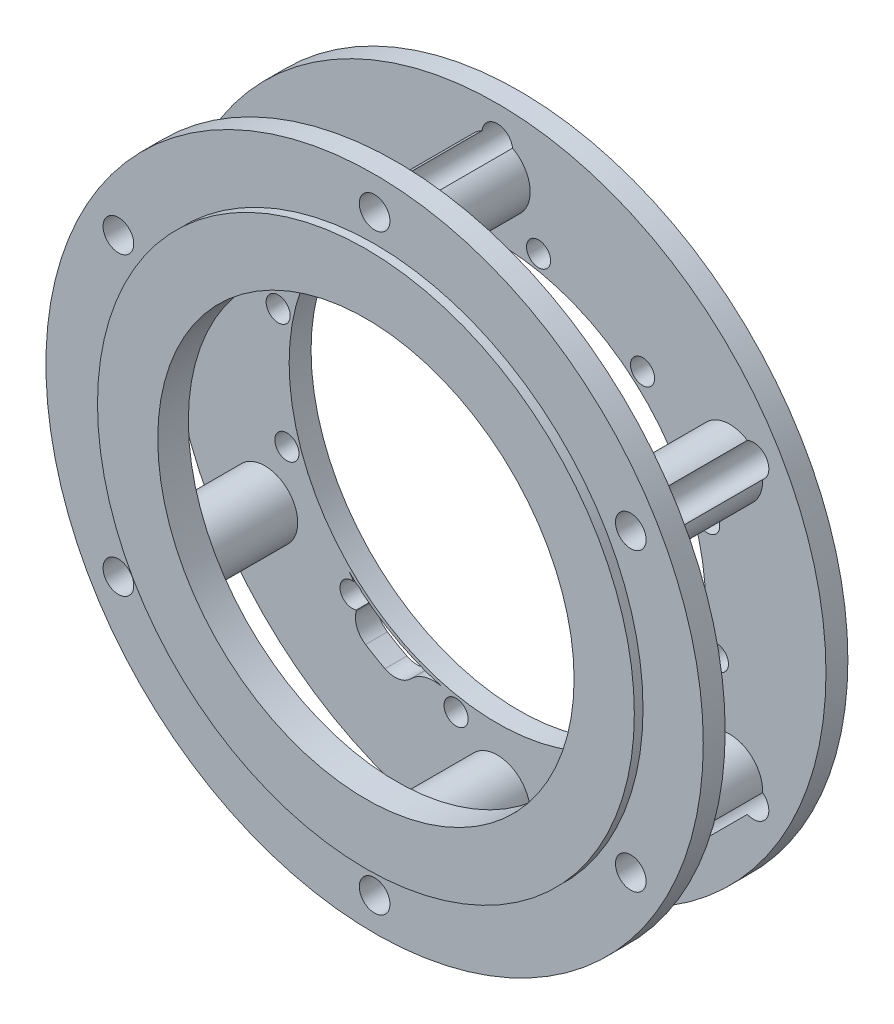
from build123d import *

# Parameters (mm, degrees)
SKETCH1_R           = 150
BOSS_EXTRUDE1_DEPTH = 10
SKETCH2_R           = 15
BOSS_EXTRUDE2_DEPTH = 46
SKETCH3_R           = 150
BOSS_EXTRUDE3_DEPTH = 10
SKETCH4_R           = 122.5
BOSS_EXTRUDE4_DEPTH = 3.96
CUT_EXTRUDE2_REACH  = 225.371
SKETCH5_R           = 7
CUT_EXTRUDE3_REACH  = 225.371
SKETCH6_R           = 95
CUT_EXTRUDE9_DEPTH  = 10
SKETCH8_R           = 5.5
CUT_EXTRUDE10_DEPTH = 10


with BuildPart() as part:
    # Sketch1 → Boss-Extrude1 (new body)
    with BuildSketch(Plane.XY):
        Circle(SKETCH1_R)
    extrude(amount=BOSS_EXTRUDE1_DEPTH)

    # Sketch2 → Boss-Extrude2 (add)
    with BuildSketch(Plane.XY.offset(10)):
        with Locations((0, 122.5)):
            Circle(SKETCH2_R)
        with Locations((106.088111964, 61.25)):
            Circle(SKETCH2_R)
        with Locations((106.088111964, -61.25)):
            Circle(SKETCH2_R)
        with Locations((0, -122.5)):
            Circle(SKETCH2_R)
        with Locations((-106.088111964, -61.25)):
            Circle(SKETCH2_R)
        with Locations((-106.088111964, 61.25)):
            Circle(SKETCH2_R)
    extrude(amount=BOSS_EXTRUDE2_DEPTH)

    # Sketch3 → Boss-Extrude3 (add)
    with BuildSketch(Plane.XY.offset(56)):
        Circle(SKETCH3_R)
    extrude(amount=BOSS_EXTRUDE3_DEPTH)

    # Sketch4 → Boss-Extrude4 (add)
    with BuildSketch(Plane.XY.offset(66)):
        Circle(SKETCH4_R)
    extrude(amount=BOSS_EXTRUDE4_DEPTH)

    # Cut-Extrude2: up to this face of the body (flat: up to its plane)
    cut_extrude2_end = Plane(part.part.faces().sort_by_distance((0, 0, 69.96))[0])
    # Sketch5 → Cut-Extrude2 (cut, up to the picked face)
    with BuildSketch(Plane(origin=(0, 0, 0), x_dir=(-1, 0, 0), z_dir=(0, 0, -1)), mode=Mode.PRIVATE) as cut_extrude2_sk1:
        with Locations((0, 135)):
            Circle(SKETCH5_R)
    cut_extrude2_tool1 = split(extrude(cut_extrude2_sk1.sketch, amount=-CUT_EXTRUDE2_REACH, mode=Mode.PRIVATE), bisect_by=cut_extrude2_end, keep=Keep.BOTH, mode=Mode.PRIVATE)
    # Sketch5 → Cut-Extrude2 (cut, up to the picked face)
    with BuildSketch(Plane(origin=(0, 0, 0), x_dir=(-1, 0, 0), z_dir=(0, 0, -1)), mode=Mode.PRIVATE) as cut_extrude2_sk2:
        with Locations((116.913429511, 67.5)):
            Circle(SKETCH5_R)
    cut_extrude2_tool2 = split(extrude(cut_extrude2_sk2.sketch, amount=-CUT_EXTRUDE2_REACH, mode=Mode.PRIVATE), bisect_by=cut_extrude2_end, keep=Keep.BOTH, mode=Mode.PRIVATE)
    # Sketch5 → Cut-Extrude2 (cut, up to the picked face)
    with BuildSketch(Plane(origin=(0, 0, 0), x_dir=(-1, 0, 0), z_dir=(0, 0, -1)), mode=Mode.PRIVATE) as cut_extrude2_sk3:
        with Locations((116.913429511, -67.5)):
            Circle(SKETCH5_R)
    cut_extrude2_tool3 = split(extrude(cut_extrude2_sk3.sketch, amount=-CUT_EXTRUDE2_REACH, mode=Mode.PRIVATE), bisect_by=cut_extrude2_end, keep=Keep.BOTH, mode=Mode.PRIVATE)
    # Sketch5 → Cut-Extrude2 (cut, up to the picked face)
    with BuildSketch(Plane(origin=(0, 0, 0), x_dir=(-1, 0, 0), z_dir=(0, 0, -1)), mode=Mode.PRIVATE) as cut_extrude2_sk4:
        with Locations((0, -135)):
            Circle(SKETCH5_R)
    cut_extrude2_tool4 = split(extrude(cut_extrude2_sk4.sketch, amount=-CUT_EXTRUDE2_REACH, mode=Mode.PRIVATE), bisect_by=cut_extrude2_end, keep=Keep.BOTH, mode=Mode.PRIVATE)
    # Sketch5 → Cut-Extrude2 (cut, up to the picked face)
    with BuildSketch(Plane(origin=(0, 0, 0), x_dir=(-1, 0, 0), z_dir=(0, 0, -1)), mode=Mode.PRIVATE) as cut_extrude2_sk5:
        with Locations((-116.913429511, -67.5)):
            Circle(SKETCH5_R)
    cut_extrude2_tool5 = split(extrude(cut_extrude2_sk5.sketch, amount=-CUT_EXTRUDE2_REACH, mode=Mode.PRIVATE), bisect_by=cut_extrude2_end, keep=Keep.BOTH, mode=Mode.PRIVATE)
    # Sketch5 → Cut-Extrude2 (cut, up to the picked face)
    with BuildSketch(Plane(origin=(0, 0, 0), x_dir=(-1, 0, 0), z_dir=(0, 0, -1)), mode=Mode.PRIVATE) as cut_extrude2_sk6:
        with Locations((-116.913429511, 67.5)):
            Circle(SKETCH5_R)
    cut_extrude2_tool6 = split(extrude(cut_extrude2_sk6.sketch, amount=-CUT_EXTRUDE2_REACH, mode=Mode.PRIVATE), bisect_by=cut_extrude2_end, keep=Keep.BOTH, mode=Mode.PRIVATE)
    add(cut_extrude2_tool1.solids().sort_by(Axis((0, 135, 0), (0, 0, 1)))[0], mode=Mode.SUBTRACT)
    add(cut_extrude2_tool2.solids().sort_by(Axis((-116.91343, 67.5, 0), (0, 0, 1)))[0], mode=Mode.SUBTRACT)
    add(cut_extrude2_tool3.solids().sort_by(Axis((-116.91343, -67.5, 0), (0, 0, 1)))[0], mode=Mode.SUBTRACT)
    add(cut_extrude2_tool4.solids().sort_by(Axis((0, -135, 0), (0, 0, 1)))[0], mode=Mode.SUBTRACT)
    add(cut_extrude2_tool5.solids().sort_by(Axis((116.91343, -67.5, 0), (0, 0, 1)))[0], mode=Mode.SUBTRACT)
    add(cut_extrude2_tool6.solids().sort_by(Axis((116.91343, 67.5, 0), (0, 0, 1)))[0], mode=Mode.SUBTRACT)

    # Cut-Extrude3: up to this face of the body (flat: up to its plane)
    cut_extrude3_end = Plane(part.part.faces().sort_by_distance((0, 0, 69.96))[0])
    # Sketch6 → Cut-Extrude3 (cut, up to the picked face)
    with BuildSketch(Plane(origin=(0, 0, 0), x_dir=(-1, 0, 0), z_dir=(0, 0, -1)), mode=Mode.PRIVATE) as cut_extrude3_sk1:
        with Locations(Location((0, 0, 0), (0, 0, 180))):
            Circle(SKETCH6_R)
    cut_extrude3_tool1 = split(extrude(cut_extrude3_sk1.sketch, amount=-CUT_EXTRUDE3_REACH, mode=Mode.PRIVATE), bisect_by=cut_extrude3_end, keep=Keep.BOTH, mode=Mode.PRIVATE)
    add(cut_extrude3_tool1.solids().sort_by(Axis((0, 0, 0), (0, 0, 1)))[0], mode=Mode.SUBTRACT)

    # Sketch7 → Cut-Extrude9 (cut)
    with BuildSketch(Plane(origin=(0, 0, 0), x_dir=(-1, 0, 0), z_dir=(0, 0, -1))):
        with BuildLine():
            ThreePointArc((68.235804385, -68.235804384), (48.250000208, -83.571451345), (24.976038317, -93.211842112))
            ThreePointArc((24.976038317, -93.211842112), (32.789258936, -93.224965512), (39.535945347, -97.165626769))
            ThreePointArc((39.535945347, -97.165626769), (45.088249404, -100.018828425), (51.250848552, -99.023232237))
            ThreePointArc((51.250848552, -99.023232237), (55.75, -96.561832522), (60.131210406, -93.89615293))
            ThreePointArc((60.131210406, -93.89615293), (64.07472157, -89.056983608), (64.379928483, -82.821946418))
            ThreePointArc((64.379928483, -82.821946418), (64.340558994, -75.008813734), (68.235804385, -68.235804384))
        make_face()
    extrude(amount=-CUT_EXTRUDE9_DEPTH, mode=Mode.SUBTRACT)

    # Sketch8 → Cut-Extrude10 (cut)
    with BuildSketch(Plane(origin=(0, 0, 0), x_dir=(-1, 0, 0), z_dir=(0, 0, -1))):
        with Locations((18.817924745, -99.994740903)):
            Circle(SKETCH8_R)
        with Locations((-33.700569576, -96.00694824)):
            Circle(SKETCH8_R)
        with Locations((-77.189023494, -66.294171327)):
            Circle(SKETCH8_R)
        with Locations((-99.994740903, -18.817924745)):
            Circle(SKETCH8_R)
        with Locations((-96.00694824, 33.700569576)):
            Circle(SKETCH8_R)
        with Locations((-66.294171327, 77.189023494)):
            Circle(SKETCH8_R)
        with Locations((-18.817924745, 99.994740903)):
            Circle(SKETCH8_R)
        with Locations((33.700569576, 96.00694824)):
            Circle(SKETCH8_R)
        with Locations((77.189023494, 66.294171327)):
            Circle(SKETCH8_R)
        with Locations((99.994740903, 18.817924745)):
            Circle(SKETCH8_R)
        with Locations((96.00694824, -33.700569576)):
            Circle(SKETCH8_R)
        with Locations((66.294171327, -77.189023494)):
            Circle(SKETCH8_R)
    extrude(amount=-CUT_EXTRUDE10_DEPTH, mode=Mode.SUBTRACT)


solid = part.part
